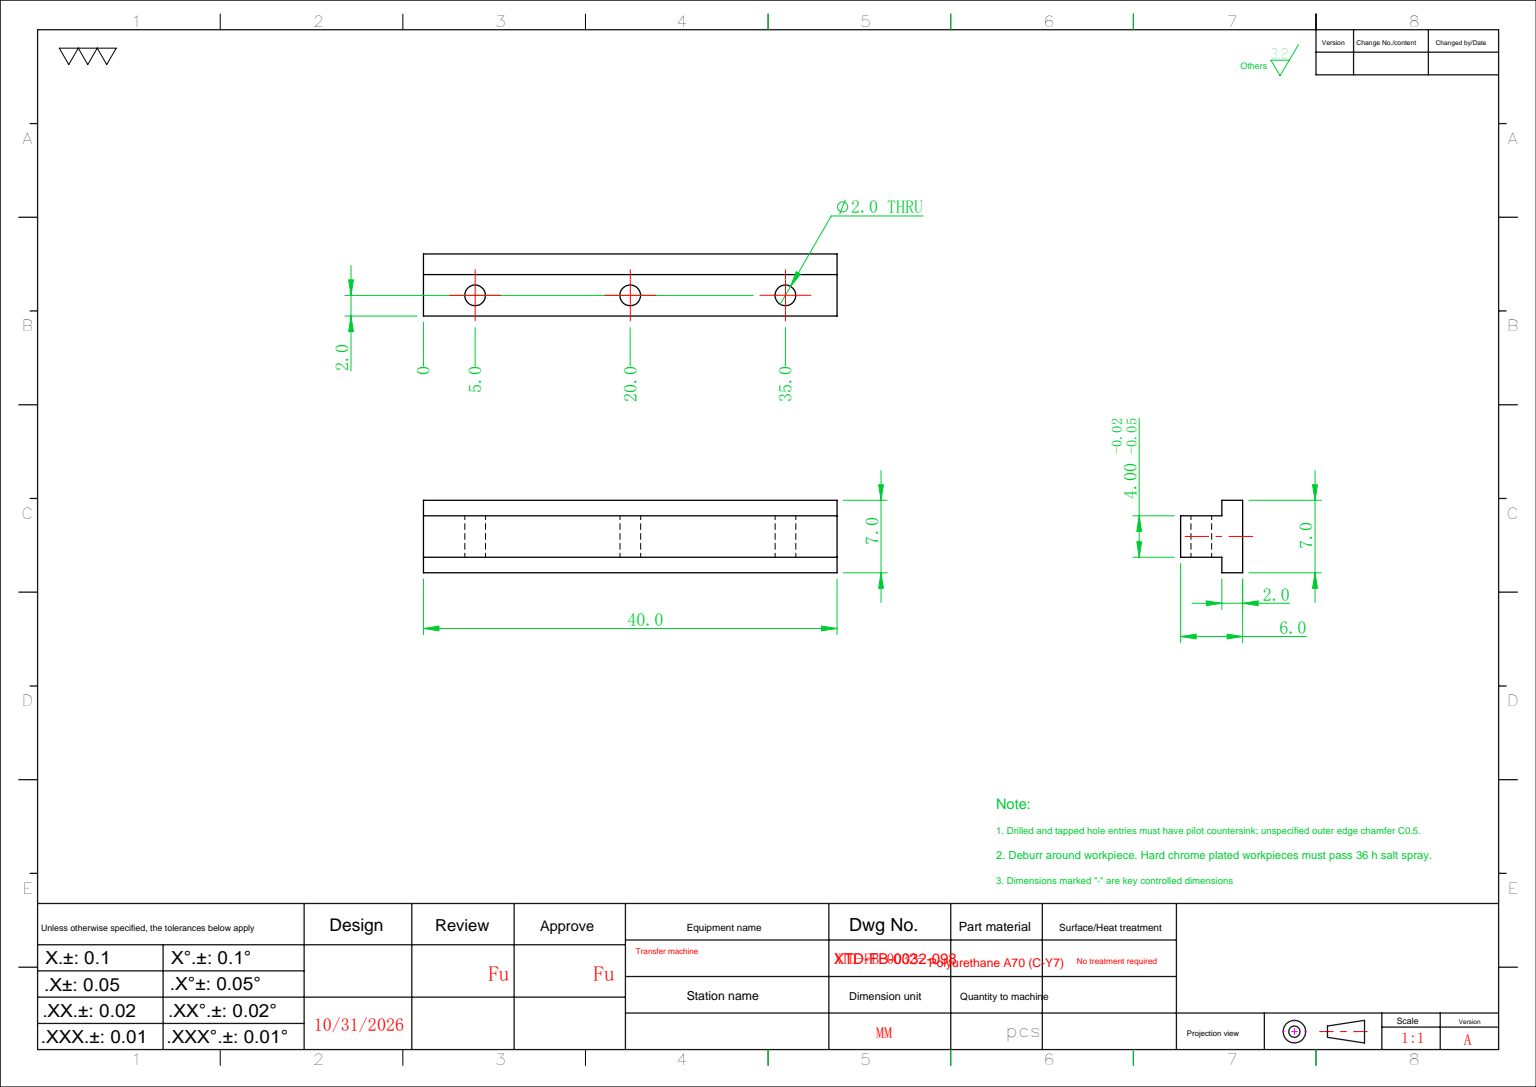
SolidWorks part; units mm, degrees
material "优力胶A70(C-Y7)"
ref_plane "前视基准面" through (0, 0, 0) normal (0, 0, 1) x (1, 0, 0)
ref_plane "上视基准面" through (0, 0, 0) normal (0, 1, 0) x (1, 0, 0)
ref_plane "右视基准面" through (0, 0, 0) normal (1, 0, 0) x (0, 0, -1)
sketch "草图1" plane through (0, 0, 0) normal (0, 0, 1) x (1, 0, 0)
  line L1 (-20, -2) -> (20, -2)
  line L2 (-20, -2) -> (-20, 2)
  line L3 (-20, 2) -> (20, 2)
  line L4 (20, -2) -> (20, 2)
  line L5 (-20, -2) -> (20, 2) construction
  line L6 (-20, 2) -> (20, -2) construction
  point P0 (0, 0)
  dimension "D1" = 4
  dimension "D2" = 40
extrude "凸台-拉伸1" add sketch "草图1" along normal blind 4
sketch "草图2" plane through (20, 0, 0) normal (1, 0, 0) x (0, 0, -1)
  line L1 (0, -3.5) -> (2, -3.5)
  line L2 (0, -3.5) -> (0, 3.5)
  line L3 (0, 3.5) -> (2, 3.5)
  line L4 (2, -3.5) -> (2, 3.5)
  line L5 (-4, 0) -> (3.959, 0) construction
  line L6 (-4, -2) -> (-4, 2) construction
  line L7 (0, -2) -> (0, 2) construction
  dimension "D1" = 2
  dimension "D2" = 7
extrude "凸台-拉伸2" add sketch "草图2" against normal up to surface (40 mm away) up to face at (-20, 0, 2)
sketch "草图3" plane through (0, 2, 0) normal (0, 1, 0) x (1, 0, 0)
  line L0 (-15, -2) -> (0, -2) construction
  line L1 (0, -2) -> (15, -2) construction
  line L2 (0, -2) -> (0, -4) construction
  line L3 (20, -4) -> (-20, -4) construction
  circle A0 centre (-15, -2) radius 1
  circle A2 centre (0, -2) radius 1
  circle A4 centre (15, -2) radius 1
  dimension "D1" = 2
  dimension "D2" = 15
  dimension "D3" = 15
  dimension "D4" = 2
extrude "切除-拉伸1" cut sketch "草图3" against normal through all
